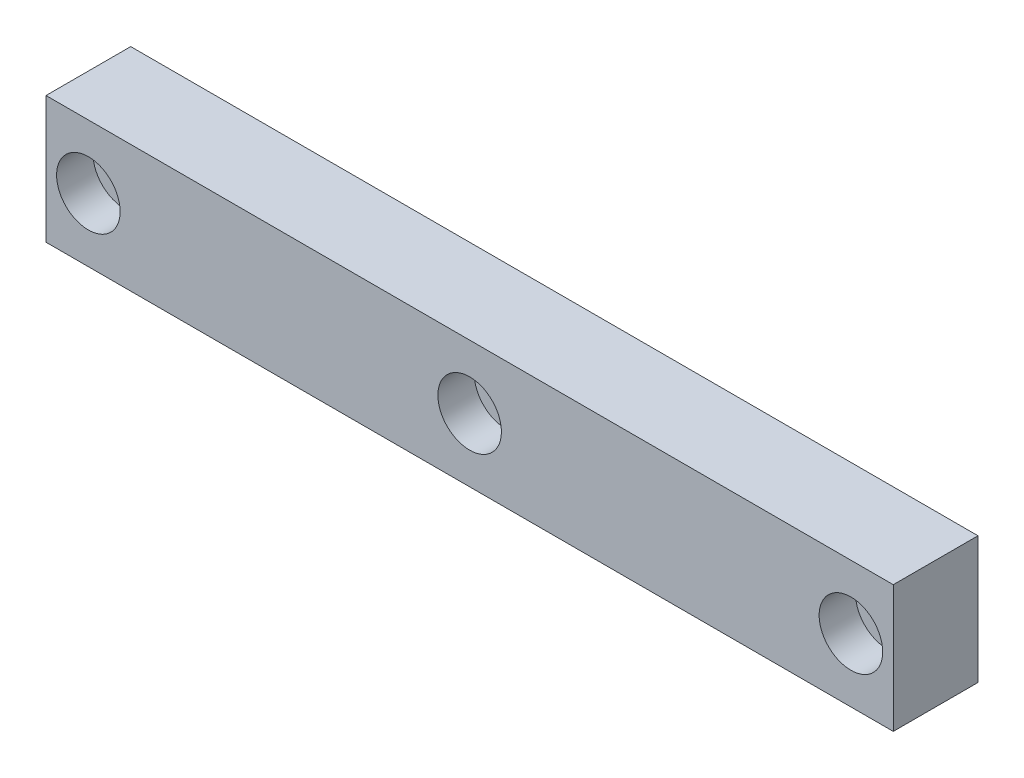
from build123d import *

# Parameters (mm, degrees)
SKETCH_1_W                   = 200
SKETCH_1_H                   = 30
EXTRUDE_1_DEPTH              = 20
HOLE_WIZARD_M8_1_D           = 9
HOLE_WIZARD_M8_1_CBORE_D     = 15
HOLE_WIZARD_M8_1_CBORE_DEPTH = 8.6


with BuildPart() as part:
    # 草图1 → 凸台-拉伸1 (new body)
    with BuildSketch(Plane.XY):
        Rectangle(SKETCH_1_W, SKETCH_1_H)
    extrude(amount=EXTRUDE_1_DEPTH)

    # M8 六角凹头螺钉的柱形沉头孔1 (through all)
    with Locations(Plane.XY.offset(20)):
        with Locations((0, 0), (90, 0), (-90, 0)):
            CounterBoreHole(HOLE_WIZARD_M8_1_D / 2, HOLE_WIZARD_M8_1_CBORE_D / 2, HOLE_WIZARD_M8_1_CBORE_DEPTH)


solid = part.part
